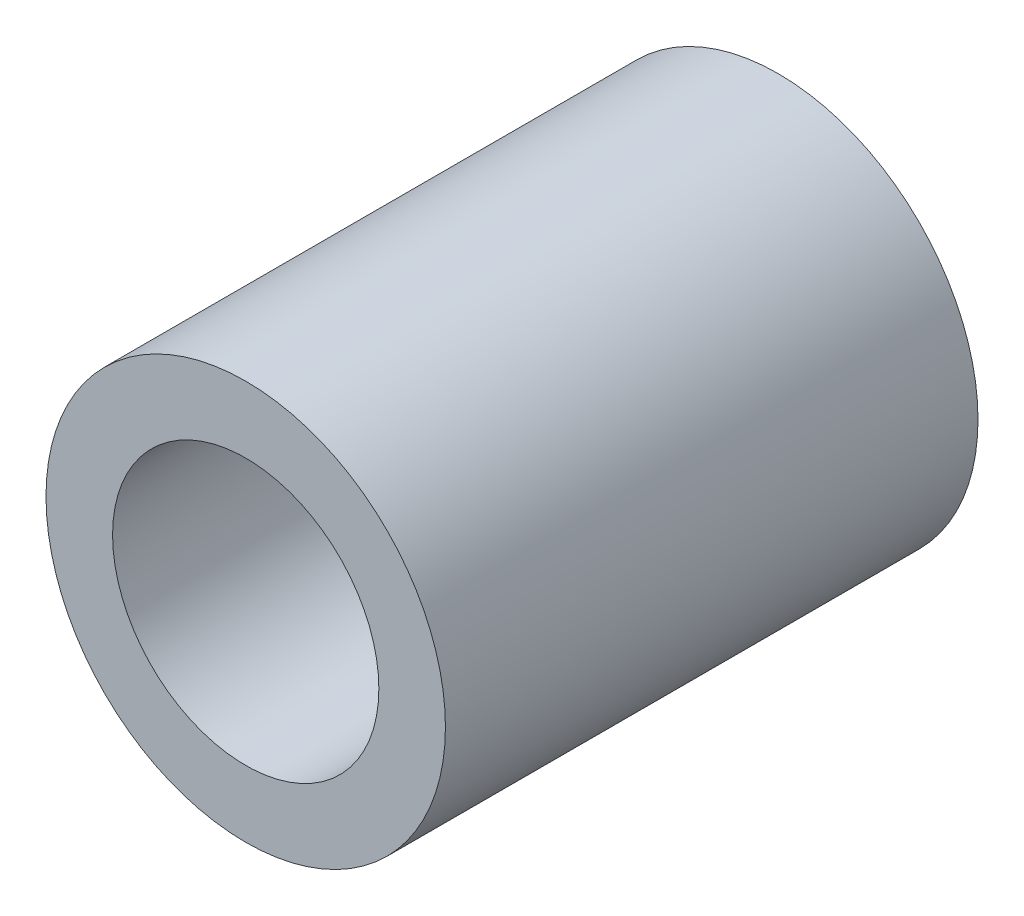
from build123d import *

# Parameters (mm, degrees)
SKETCH2_R           = 7.5
SKETCH2_R_2         = 5
BOSS_EXTRUDE1_DEPTH = 10


with BuildPart() as part:
    # Sketch2 → Boss-Extrude1 (new, symmetric)
    with BuildSketch(Plane.XY):
        Circle(SKETCH2_R)
        Circle(SKETCH2_R_2, mode=Mode.SUBTRACT)
    extrude(amount=BOSS_EXTRUDE1_DEPTH, both=True)


solid = part.part
